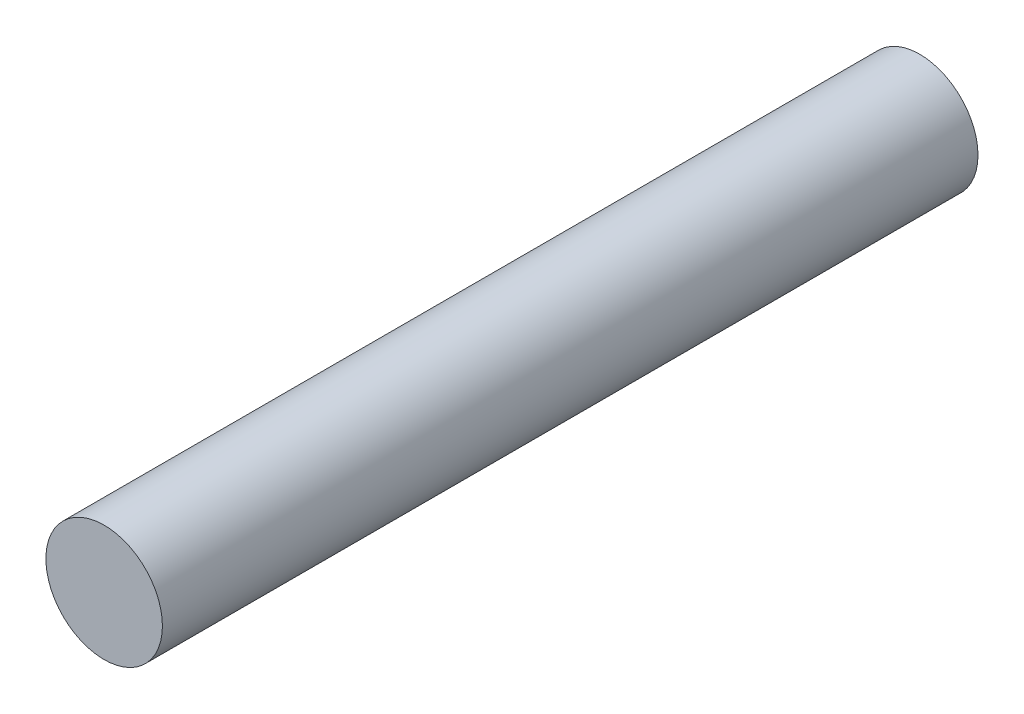
SolidWorks part; units mm, degrees
ref_plane "Front Plane" through (0, 0, 0) normal (0, 0, 1) x (1, 0, 0)
ref_plane "Top Plane" through (0, 0, 0) normal (0, 1, 0) x (1, 0, 0)
ref_plane "Right Plane" through (0, 0, 0) normal (1, 0, 0) x (0, 0, -1)
other "Configuration Table"
sketch "Sketch1" plane through (0, 0, 0) normal (0, 0, 1) x (1, 0, 0)
  circle A0 centre (0, 0) radius 20
extrude "Boss-Extrude1" add sketch "Sketch1" against normal blind 30 and the other way blind 250
